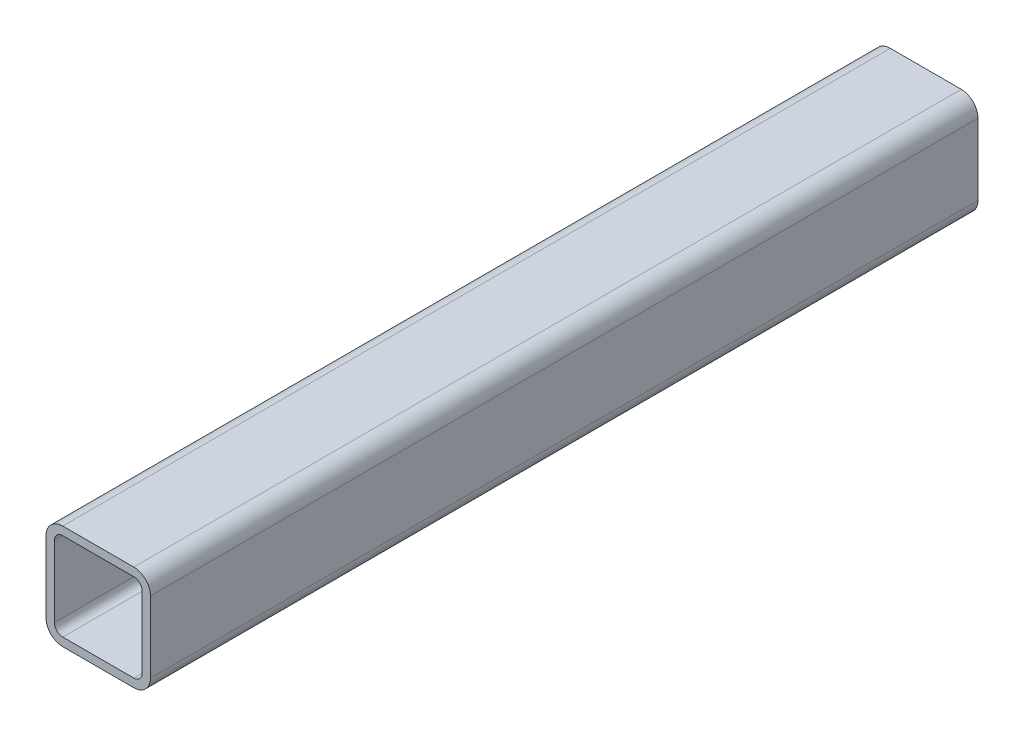
from build123d import *

# Parameters (mm, degrees)
BOSS_EXTRUDE1_DEPTH = 198


with BuildPart() as part:
    # Sketch1 → Boss-Extrude1 (new body)
    with BuildSketch(Plane.XY):
        with BuildLine():
            Line((-8.5, -12.5), (8.5, -12.5))
            ThreePointArc((8.5, -12.5), (11.328427125, -11.328427125), (12.5, -8.5))
            Line((12.5, -8.5), (12.5, 8.5))
            ThreePointArc((12.5, 8.5), (11.328427125, 11.328427125), (8.5, 12.5))
            Line((8.5, 12.5), (-8.5, 12.5))
            ThreePointArc((-8.5, 12.5), (-11.328427125, 11.328427125), (-12.5, 8.5))
            Line((-12.5, 8.5), (-12.5, -8.5))
            ThreePointArc((-12.5, -8.5), (-11.328427125, -11.328427125), (-8.5, -12.5))
        make_face()
        with BuildLine():
            Line((-8.5, -10.5), (8.5, -10.5))
            ThreePointArc((8.5, -10.5), (9.914213562, -9.914213562), (10.5, -8.5))
            Line((10.5, -8.5), (10.5, 8.5))
            ThreePointArc((10.5, 8.5), (9.914213562, 9.914213562), (8.5, 10.5))
            Line((8.5, 10.5), (-8.5, 10.5))
            ThreePointArc((-8.5, 10.5), (-9.914213562, 9.914213562), (-10.5, 8.5))
            Line((-10.5, 8.5), (-10.5, -8.5))
            ThreePointArc((-10.5, -8.5), (-9.914213562, -9.914213562), (-8.5, -10.5))
        make_face(mode=Mode.SUBTRACT)
    extrude(amount=BOSS_EXTRUDE1_DEPTH)


solid = part.part
